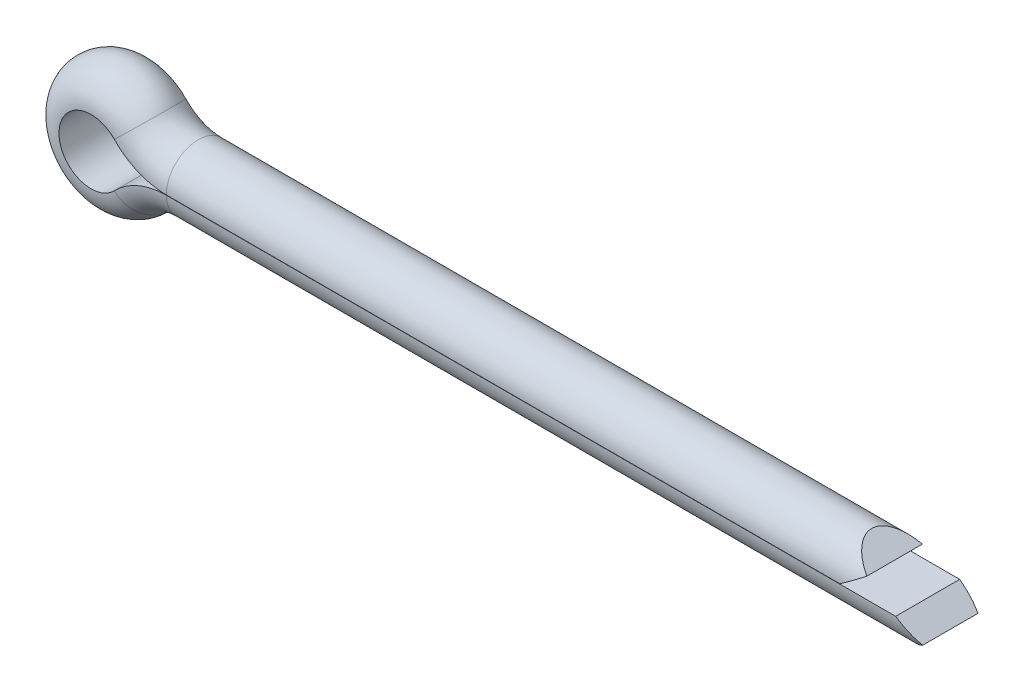
from build123d import *

# Parameters (mm, degrees)
CUT_EXTRUDE_1_DEPTH      = 60.622226572
CUT_EXTRUDE_1_DEPTH_BACK = 60.622226572


with BuildPart() as part:
    # 扫描2: sweep along a path in Sketch 203
    with BuildLine(Plane.XY) as sweep_2_path:
        Line((55.4, 2.3), (5.4, 2.3))
        ThreePointArc((5.4, 2.3), (4.267859381, 2.531061156), (3.316806967, 3.187285922))
        ThreePointArc((3.316806967, 3.187285922), (-4.6, 0), (3.316806967, -3.187285922))
        ThreePointArc((3.316806967, -3.187285922), (4.267859381, -2.531061156), (5.4, -2.3))
        Line((5.4, -2.3), (59.4, -2.3))
    # 草图2 → 扫描2 (sweep)
    with BuildSketch(Plane(origin=(55.4, 2.3, 0), x_dir=(0, 0, 1), z_dir=(-1, 0, 0))):
        with BuildLine():
            Line((-2.299978261, -2.29), (2.299978261, -2.29))
            ThreePointArc((2.299978261, -2.29), (0, 0), (-2.299978261, -2.29))
        make_face()
    sweep(path=sweep_2_path.line)

    # 草图3 → 切除-拉伸1 (cut, two sides: drawn at the far end of the back side and taken through both)
    with BuildSketch(Plane.XY.offset(-CUT_EXTRUDE_1_DEPTH_BACK)):
        Polygon((55.4, 1.145), (53.76113083, 2.3), (59.41, 2.3), (59.41, -2.3), (57.754128755, -2.3), (59.4, -1.155), (57.76113083, 0), (53.754128755, 0), align=None)
    extrude(amount=CUT_EXTRUDE_1_DEPTH + CUT_EXTRUDE_1_DEPTH_BACK, mode=Mode.SUBTRACT)


solid = part.part
